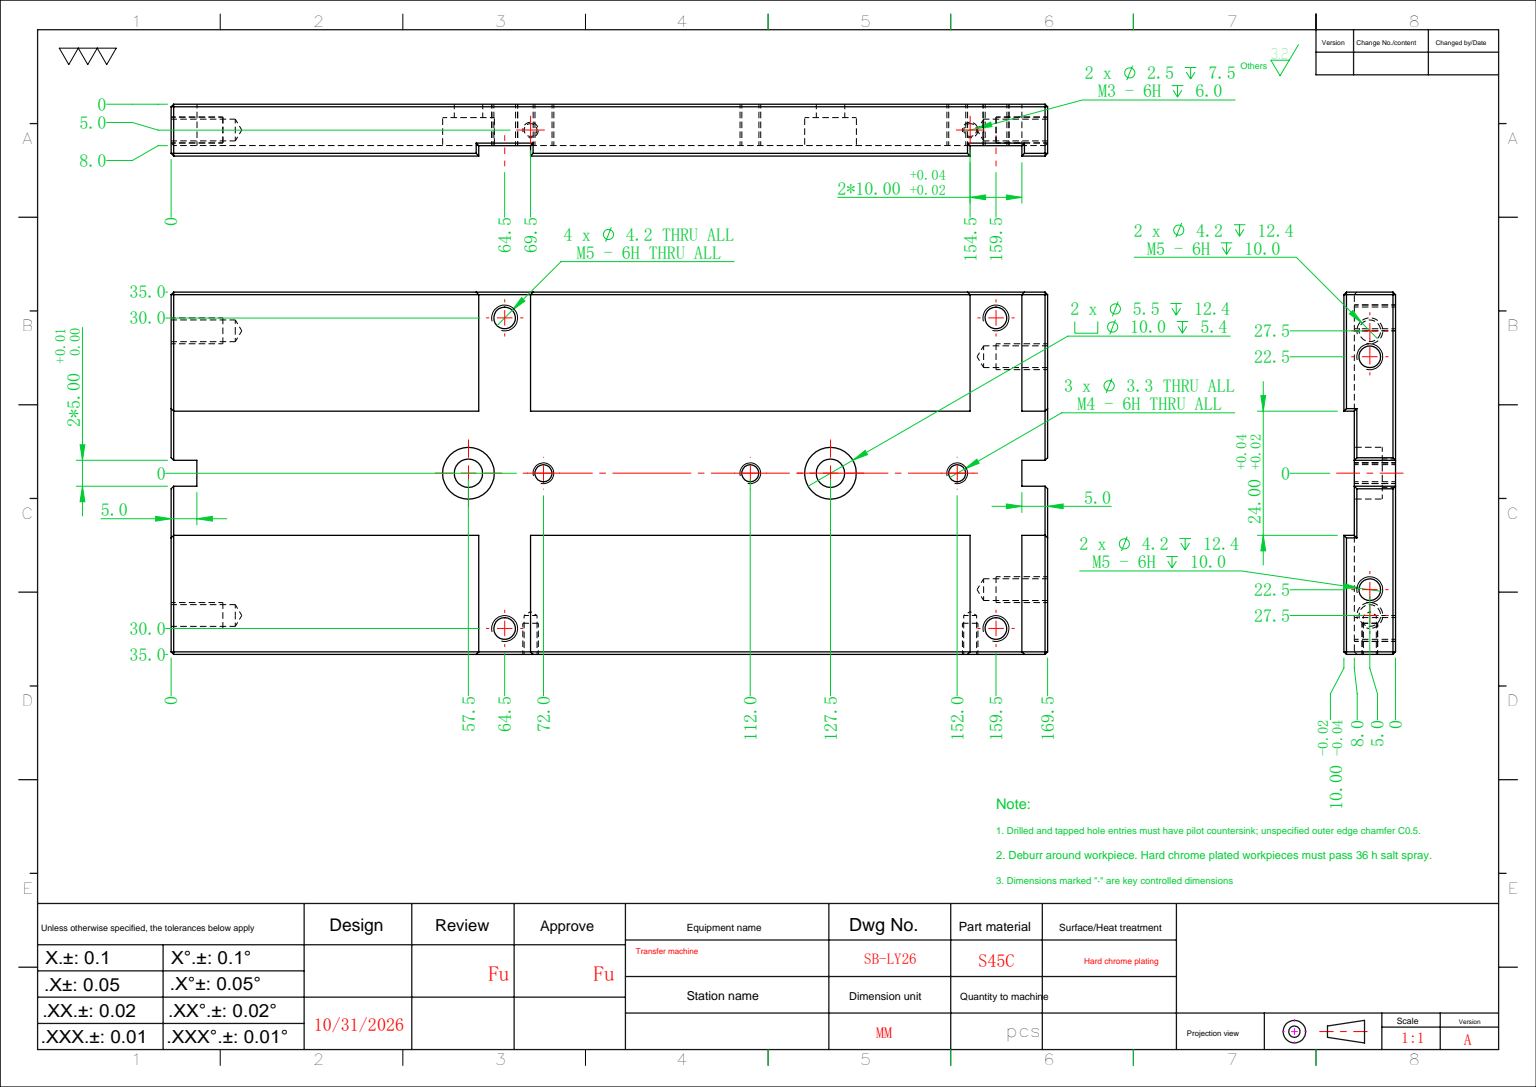
SolidWorks part; units mm, degrees
ref_plane "前视基准面" through (0, 0, 0) normal (0, 0, 1) x (1, 0, 0)
ref_plane "上视基准面" through (0, 0, 0) normal (0, 1, 0) x (1, 0, 0)
ref_plane "右视基准面" through (0, 0, 0) normal (1, 0, 0) x (0, 0, -1)
sketch "草图1" plane through (0, 0, 0) normal (0, 0, 1) x (1, 0, 0)
  line L1 (-35, -84.75) -> (35, -84.75)
  line L2 (-35, -84.75) -> (-35, 84.75)
  line L3 (-35, 84.75) -> (35, 84.75)
  line L4 (35, -84.75) -> (35, 84.75)
  line L5 (-35, -84.75) -> (35, 84.75) construction
  line L6 (-35, 84.75) -> (35, -84.75) construction
  point P0 (0, 0)
  dimension "D1" = 70
  dimension "D2" = 169.5
extrude "凸台-拉伸1" add sketch "草图1" along normal blind 10
sketch "草图2" plane through (0, -84.75, 0) normal (0, -1, 0) x (1, 0, 0)
  line L0 (-35, 0) -> (35, 0) construction
  line L1 (12, 0) -> (-12, 0)
  line L2 (12, 0) -> (12, 2)
  line L3 (12, 2) -> (-12, 2)
  line L4 (-12, 0) -> (-12, 2)
  line L5 (0, 0) -> (0, 7.707) construction
  dimension "D1" = 24
  dimension "D2" = 2
extrude "切除-拉伸1" cut sketch "草图2" against normal through all
sketch "草图3" plane through (0, 0, 0) normal (0, 0, -1) x (-1, 0, 0)
  line L0 (35, 84.75) -> (35, -84.75) construction
  line L1 (35, 69.75) -> (-35, 69.75)
  line L2 (35, 69.75) -> (35, 79.75)
  line L3 (35, 79.75) -> (-35, 79.75)
  line L4 (-35, 69.75) -> (-35, 79.75)
  line L5 (-35, -84.75) -> (-35, 84.75) construction
  line L6 (35, 74.75) -> (9.6921, 74.75) construction
  line L7 (-35, 84.75) -> (35, 84.75) construction
  dimension "D1" = 10
  dimension "D2" = 10
extrude "切除-拉伸2" cut sketch "草图3" against normal up to surface (2 mm away) up to face at (0, 0, 2)
sketch "草图4" plane through (0, 0, 0) normal (0, 0, -1) x (-1, 0, 0)
  line L0 (35, 69.75) -> (35, -84.75) construction
  line L1 (35, -25.25) -> (-35, -25.25)
  line L2 (35, -25.25) -> (35, -15.25)
  line L3 (35, -15.25) -> (-35, -15.25)
  line L4 (-35, -25.25) -> (-35, -15.25)
  line L5 (-35, -84.75) -> (-35, 69.75) construction
  line L8 (35, -20.25) -> (37.2552, -20.25) construction
  line L9 (35, 79.75) -> (12, 79.75) construction
  dimension "D1" = 95
  dimension "D2" = 10
extrude "切除-拉伸3" cut sketch "草图4" against normal up to surface (2 mm away) up to face at (0, 49.8333, 2)
hole_wizard "M5 螺纹孔1" positions "草图5" profile "草图6" tap size "M5" standard "ISO" end condition through all
sketch "草图5" plane through (0, 0, 0) normal (0, 0, -1) x (-1, 0, 0)
  line L0 (-35, 74.75) -> (35, 74.75) construction
  line L1 (-35, 79.75) -> (-35, 69.75) construction
  line L2 (35, 69.75) -> (35, 79.75) construction
  line L4 (0, 84.75) -> (0, -84.9426) construction
  line L5 (-12, 84.75) -> (12, 84.75) construction
  line L7 (35, -20.25) -> (-35, -20.25) construction
  line L8 (35, -25.25) -> (35, -15.25) construction
  line L9 (-35, -15.25) -> (-35, -25.25) construction
  point P0 (-30, -20.25)
  point P3 (30, -20.25)
  point P6 (-30, 74.75)
  point P9 (30, 74.75)
  dimension "D1" = 60
sketch "草图6" plane through (30, -20.25, 0) normal (1, 0, 0) x (0, 1, 0)
  line L0 (0, 0) -> (0, 10)
  line L1 (0, 10) -> (2.1, 10)
  line L2 (2.1, 10) -> (2.1, 0)
  line L5 (2.1, 0) -> (0, 0)
  line L11 (0, -6.35) -> (0, 107.95) construction
  dimension "通孔螺纹孔钻头直径" = 4.2
  dimension "通孔螺纹孔钻头深度" = 10
cosmetic thread "孔螺蚊线1" parameters "D2"=5
cosmetic thread "孔螺蚊线2" parameters "D2"=5
cosmetic thread "孔螺蚊线3" parameters "D2"=5
cosmetic thread "孔螺蚊线4" parameters "D2"=5
hole_wizard "M4 螺纹孔1" positions "草图7" profile "草图8" tap size "M4" standard "ISO" end condition through all
sketch "草图7" plane through (0, 0, 2) normal (0, 0, -1) x (-1, 0, 0)
  line L0 (0, 84.75) -> (0, -30.2197) construction
  line L1 (-12, 84.75) -> (12, 84.75) construction
  line L3 (-35, 84.75) -> (35, 84.75) construction
  point P0 (0, -12.75)
  point P3 (0, 27.25)
  point P6 (0, 67.25)
  dimension "D1" = 17.5
  dimension "D2" = 40
  dimension "D3" = 40
sketch "草图8" plane through (0, -12.75, 2) normal (1, 0, 0) x (0, 1, 0)
  line L0 (0, 0) -> (0, 8)
  line L1 (0, 8) -> (1.65, 8)
  line L2 (1.65, 8) -> (1.65, 0)
  line L5 (1.65, 0) -> (0, 0)
  line L11 (0, -6.35) -> (0, 107.95) construction
  dimension "通孔螺纹孔钻头直径" = 3.3
  dimension "通孔螺纹孔钻头深度" = 8
cosmetic thread "孔螺蚊线5" parameters "D2"=4
cosmetic thread "孔螺蚊线6" parameters "D2"=4
cosmetic thread "孔螺蚊线7" parameters "D2"=4
hole_wizard "M5 螺纹孔2" positions "草图9" profile "草图10" tap size "M5" standard "ISO"
sketch "草图9" plane through (0, -84.75, 0) normal (0, -1, 0) x (-1, 0, 0)
  line L0 (0, 0) -> (0, -10) construction
  line L1 (35, -10) -> (-35, -10) construction
  line L3 (35, -5) -> (-35, -5) construction
  line L4 (35, -10) -> (35, 0) construction
  line L5 (-35, -10) -> (-35, 0) construction
  point P0 (-27.5, -5)
  point P3 (27.5, -5)
  dimension "D1" = 55
sketch "草图10" plane through (27.5, -84.75, 5) normal (1, 0, 0) x (0, 0, -1)
  line L0 (0, 0) -> (0, 13.6618)
  line L1 (0, 13.6618) -> (2.1, 12.4)
  line L2 (2.1, 12.4) -> (2.1, 0)
  line L5 (2.1, 0) -> (0, 0)
  line L10 (0, 13.6618) -> (-2.1, 12.4) construction
  line L11 (0, -6.35) -> (0, 107.95) construction
  dimension "螺纹孔钻头直径" = 4.2
  dimension "螺纹孔钻头深度" = 12.4
  dimension "导头角度" = 118
cosmetic thread "孔螺蚊线8" parameters "D1"=10, "D2"=5
cosmetic thread "孔螺蚊线9" parameters "D1"=10, "D2"=5
sketch "草图11" plane through (0, -84.75, 0) normal (0, -1, 0) x (1, 0, 0)
  line L0 (-35, 10) -> (35, 10) construction
  line L1 (-2.5, 10) -> (2.5, 10)
  line L2 (-2.5, 10) -> (-2.5, 2)
  line L3 (-2.5, 2) -> (2.5, 2)
  line L4 (2.5, 10) -> (2.5, 2)
  line L5 (0, 10) -> (0, -6.8209) construction
  line L6 (12, 2) -> (-12, 2) construction
  dimension "D1" = 5
extrude "切除-拉伸4" cut sketch "草图11" against normal blind 5
hole_wizard "M5 螺纹孔3" positions "草图12" profile "草图13" tap size "M5" standard "ISO"
sketch "草图12" plane through (0, 84.75, 0) normal (0, 1, 0) x (1, 0, 0)
  line L0 (0, -10) -> (0, 3.7334) construction
  line L1 (35, -10) -> (-35, -10) construction
  line L3 (35, -5) -> (-35, -5) construction
  line L4 (35, -10) -> (35, 0) construction
  line L5 (-35, -10) -> (-35, 0) construction
  point P0 (22.5, -5)
  point P3 (-22.5, -5)
  dimension "D1" = 45
sketch "草图13" plane through (22.5, 84.75, 5) normal (1, 0, 0) x (0, 0, 1)
  line L0 (0, 0) -> (0, 13.6618)
  line L1 (0, 13.6618) -> (2.1, 12.4)
  line L2 (2.1, 12.4) -> (2.1, 0)
  line L5 (2.1, 0) -> (0, 0)
  line L10 (0, 13.6618) -> (-2.1, 12.4) construction
  line L11 (0, -6.35) -> (0, 107.95) construction
  dimension "螺纹孔钻头直径" = 4.2
  dimension "螺纹孔钻头深度" = 12.4
  dimension "导头角度" = 118
cosmetic thread "孔螺蚊线10" parameters "D1"=10, "D2"=5
cosmetic thread "孔螺蚊线11" parameters "D1"=10, "D2"=5
sketch "草图14" plane through (0, 84.75, 0) normal (0, 1, 0) x (1, 0, 0)
  line L0 (12, -2) -> (-12, -2) construction
  line L1 (-2.5, -2) -> (2.5, -2)
  line L2 (-2.5, -2) -> (-2.5, -10)
  line L3 (-2.5, -10) -> (2.5, -10)
  line L4 (2.5, -2) -> (2.5, -10)
  line L5 (35, -10) -> (-35, -10) construction
  line L6 (0, -10) -> (0, 7.2336) construction
  dimension "D1" = 5
extrude "切除-拉伸5" cut sketch "草图14" against normal blind 5
hole_wizard "M5 六角凹头螺钉的柱形沉头孔1" positions "草图15" profile "草图16" counterbore size "M5" standard "ISO"
sketch "草图15" plane through (0, 0, 2) normal (0, 0, -1) x (-1, 0, 0)
  line L0 (0, 0) -> (0, 92.3826) construction
  line L2 (5, 82.75) -> (-5, 82.75) construction
  point P0 (0, -27.25)
  point P2 (0, 42.75)
  dimension "D1" = 70
  dimension "D2" = 40
sketch "草图16" plane through (0, -27.25, 2) normal (1, 0, 0) x (0, 1, 0)
  line L0 (0, 0) -> (0, 14.0524)
  line L1 (0, 14.0524) -> (2.75, 12.4)
  line L2 (2.75, 12.4) -> (2.75, 5.4)
  line L3 (2.75, 5.4) -> (5, 5.4)
  line L4 (5, 5.4) -> (5, 0)
  line L5 (5, 0) -> (0, 0)
  line L10 (0, 14.0524) -> (-2.75, 12.4) construction
  line L11 (0, -6.35) -> (0, 107.95) construction
  dimension "孔直径" = 5.5
  dimension "孔深度" = 12.4
  dimension "柱形沉头孔直径" = 10
  dimension "柱形沉头孔深度" = 5.4
  dimension "导头角度" = 118
hole_wizard "M3 螺纹孔1" positions "草图17" profile "草图18" tap size "M3" standard "ISO"
sketch "草图17" plane through (-35, 0, 0) normal (-1, 0, 0) x (0, 0, 1)
  line L0 (5, -84.75) -> (5, 84.75) construction
  line L1 (10, -84.75) -> (0, -84.75) construction
  line L2 (10, 84.75) -> (0, 84.75) construction
  point P0 (5, -15.25)
  point P3 (5, 69.75)
  dimension "D1" = 85
  dimension "D2" = 15
sketch "草图18" plane through (-35, -15.25, 5) normal (0, 1, 0) x (0, 0, 1)
  line L0 (0, 0) -> (0, 8.2511)
  line L1 (0, 8.2511) -> (1.25, 7.5)
  line L2 (1.25, 7.5) -> (1.25, 0)
  line L5 (1.25, 0) -> (0, 0)
  line L10 (0, 8.2511) -> (-1.25, 7.5) construction
  line L11 (0, -6.35) -> (0, 107.95) construction
  dimension "螺纹孔钻头直径" = 2.5
  dimension "螺纹孔钻头深度" = 7.5
  dimension "导头角度" = 118
cosmetic thread "孔螺蚊线12" parameters "D1"=6, "D2"=3
cosmetic thread "孔螺蚊线13" parameters "D1"=6, "D2"=3
chamfer "倒角1" distance 0.5 angle 45 44 edges at (35, -25.25, 1) (35, -55, 0) (35, -20.25, 2) (35, -15.25, 1) (35, 27.25, 0) (35, 69.75, 1) (35, 74.75, 2) (35, 79.75, 1) (35, 82.25, 0) (12, 84.75, 1) (23.5, 84.75, 0) (35, 84.75, 5) (7.25, 84.75, 2) (2.5, 84.75, 6) (18.75, 84.75, 10) (35, 0, 10) (35, -84.75, 5) (23.5, -84.75, 0) (12, -84.75, 1) (7.25, -84.75, 2) (2.5, -84.75, 6) (18.75, -84.75, 10) (-23.5, 84.75, 0) (-12, 84.75, 1) (-7.25, 84.75, 2) (-2.5, 84.75, 6) (-18.75, 84.75, 10) (-35, 69.75, 1) (-35, 74.75, 2) (-35, 79.75, 1) (-35, 82.25, 0) (-35, 84.75, 5) (-35, 0, 10) (-35, 27.25, 0) (-35, -15.25, 1) (-35, -20.25, 2) (-35, -25.25, 1) (-35, -55, 0) (-12, -84.75, 1) (-23.5, -84.75, 0) (-35, -84.75, 5) (-18.75, -84.75, 10) (-2.5, -84.75, 6) (-7.25, -84.75, 2)
